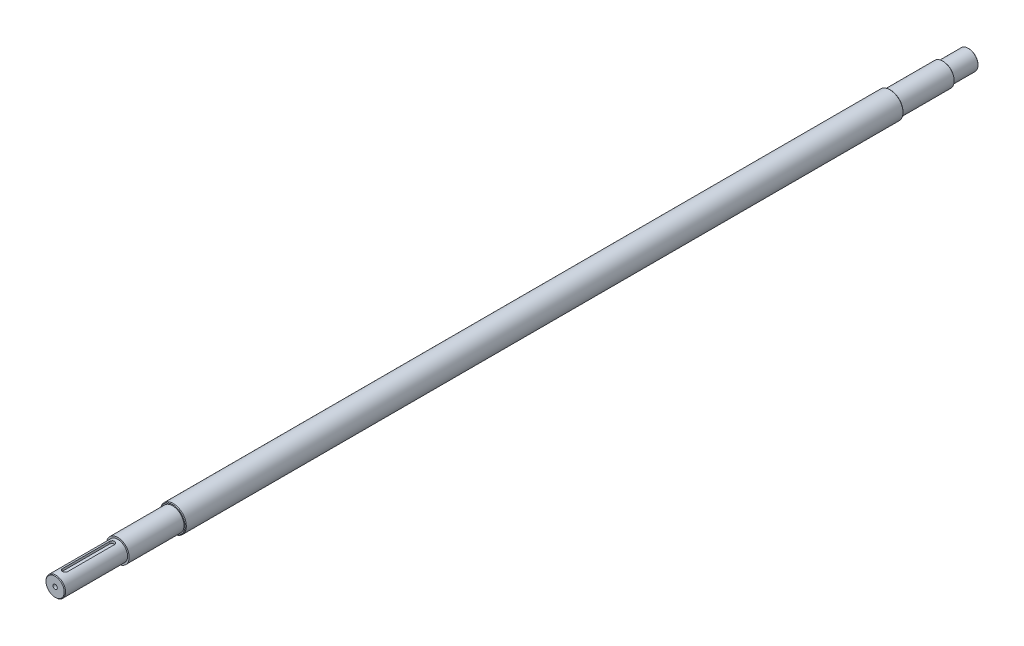
SolidWorks part; units mm, degrees
ref_plane "前视基准面" through (0, 0, 0) normal (0, 0, 1) x (1, 0, 0)
ref_plane "上视基准面" through (0, 0, 0) normal (0, 1, 0) x (1, 0, 0)
ref_plane "右视基准面" through (0, 0, 0) normal (1, 0, 0) x (0, 0, -1)
sketch "草图2" plane through (0, 0, 0) normal (0, 0, 1) x (1, 0, 0)
  circle A0 centre (0, 0) radius 15
  dimension "D1" = 30
extrude "凸台-拉伸1" add sketch "草图2" against normal blind 96
sketch "草图3" plane through (0, 0, -96) normal (0, 0, -1) x (-1, 0, 0)
  circle A0 centre (0, 0) radius 17.5
  dimension "D1" = 35
extrude "凸台-拉伸2" add sketch "草图3" along normal blind 84
sketch "草图4" plane through (0, 0, -180) normal (0, 0, -1) x (-1, 0, 0)
  circle A0 centre (0, 0) radius 20
  dimension "D1" = 40
extrude "凸台-拉伸3" add sketch "草图4" along normal blind 1100
sketch "草图6" plane through (0, 0, -1280) normal (0, 0, -1) x (-1, 0, 0)
  circle A0 centre (0, 0) radius 17.5
  dimension "D1" = 35
extrude "凸台-拉伸4" add sketch "草图6" along normal blind 80
sketch "草图7" plane through (0, 0, -1360) normal (0, 0, -1) x (-1, 0, 0)
  circle A0 centre (0, 0) radius 13
  dimension "D1" = 26
extrude "凸台-拉伸5" add sketch "草图7" along normal blind 2
sketch "草图9" plane through (0, 0, -1362) normal (0, 0, -1) x (-1, 0, 0)
  circle A0 centre (0, 0) radius 15
  dimension "D1" = 30
extrude "凸台-拉伸6" add sketch "草图9" along normal blind 38
cosmetic thread "装饰螺纹线1" parameters "D2"=29
chamfer "倒角1" distance 1 angle 45 1 edges at (-15, 0, -1400)
chamfer "倒角2" distance 1 angle 45 1 edges at (-20, 0, -1280)
chamfer "倒角3" distance 1 angle 45 1 edges at (-20, 0, -180)
chamfer "倒角4" distance 1 angle 45 1 edges at (15, 0, 0)
sketch "草图11" plane through (0, 0, 0) normal (0, 0, 1) x (1, 0, 0)
  point P0 (0, 0)
move or copy body "实体-移动/复制1" bodies to move or copy 111 copy no translate (0, 0, 10)
hole_wizard "M8 螺纹孔2" positions "3D草图6" profile "草图16" tap size "M8" standard "GB"
sketch3d "3D草图6"
  line L0 (0, 0, 9) -> (0, 0, 10) construction
  point P0 (0, 0, 10)
sketch "草图16" plane through (0, 0, 10) normal (1, 0, 0) x (0, -1, 0)
  line L0 (0, 0) -> (0, 30.7929)
  line L1 (0, 30.7929) -> (3.4, 28.75)
  line L2 (3.4, 28.75) -> (3.4, 0)
  line L5 (3.4, 0) -> (0, 0)
  line L10 (0, 30.7929) -> (-3.4, 28.75) construction
  line L11 (0, -6.35) -> (0, 107.95) construction
  dimension "螺纹孔钻头直径" = 6.8
  dimension "螺纹孔钻头深度" = 28.75
  dimension "导头角度" = 118
cosmetic thread "孔螺蚊线2" parameters "D1"=25, "D2"=8
ref_plane "基准面1" through (0, 11, 0) normal (0, 1, 0) x (1, 0, 0)
sketch "草图18" plane through (0, 11, 0) normal (0, 1, 0) x (1, 0, 0)
  line L0 (0, 77) -> (0, 5) construction
  line L1 (4, 77) -> (4, 5)
  line L2 (-4, 77) -> (-4, 5)
  line L3 (-17.5, 86) -> (17.5, 86) construction
  arc A0 (4, 77) -> (-4, 77) centre (0, 77) ccw
  arc A1 (-4, 5) -> (4, 5) centre (0, 5) ccw
  point P3 (0, 41)
  dimension "D2" = 5
  dimension "D3" = 80
  dimension "D1" = 8
extrude "切除-拉伸1" cut sketch "草图18" along normal through all
